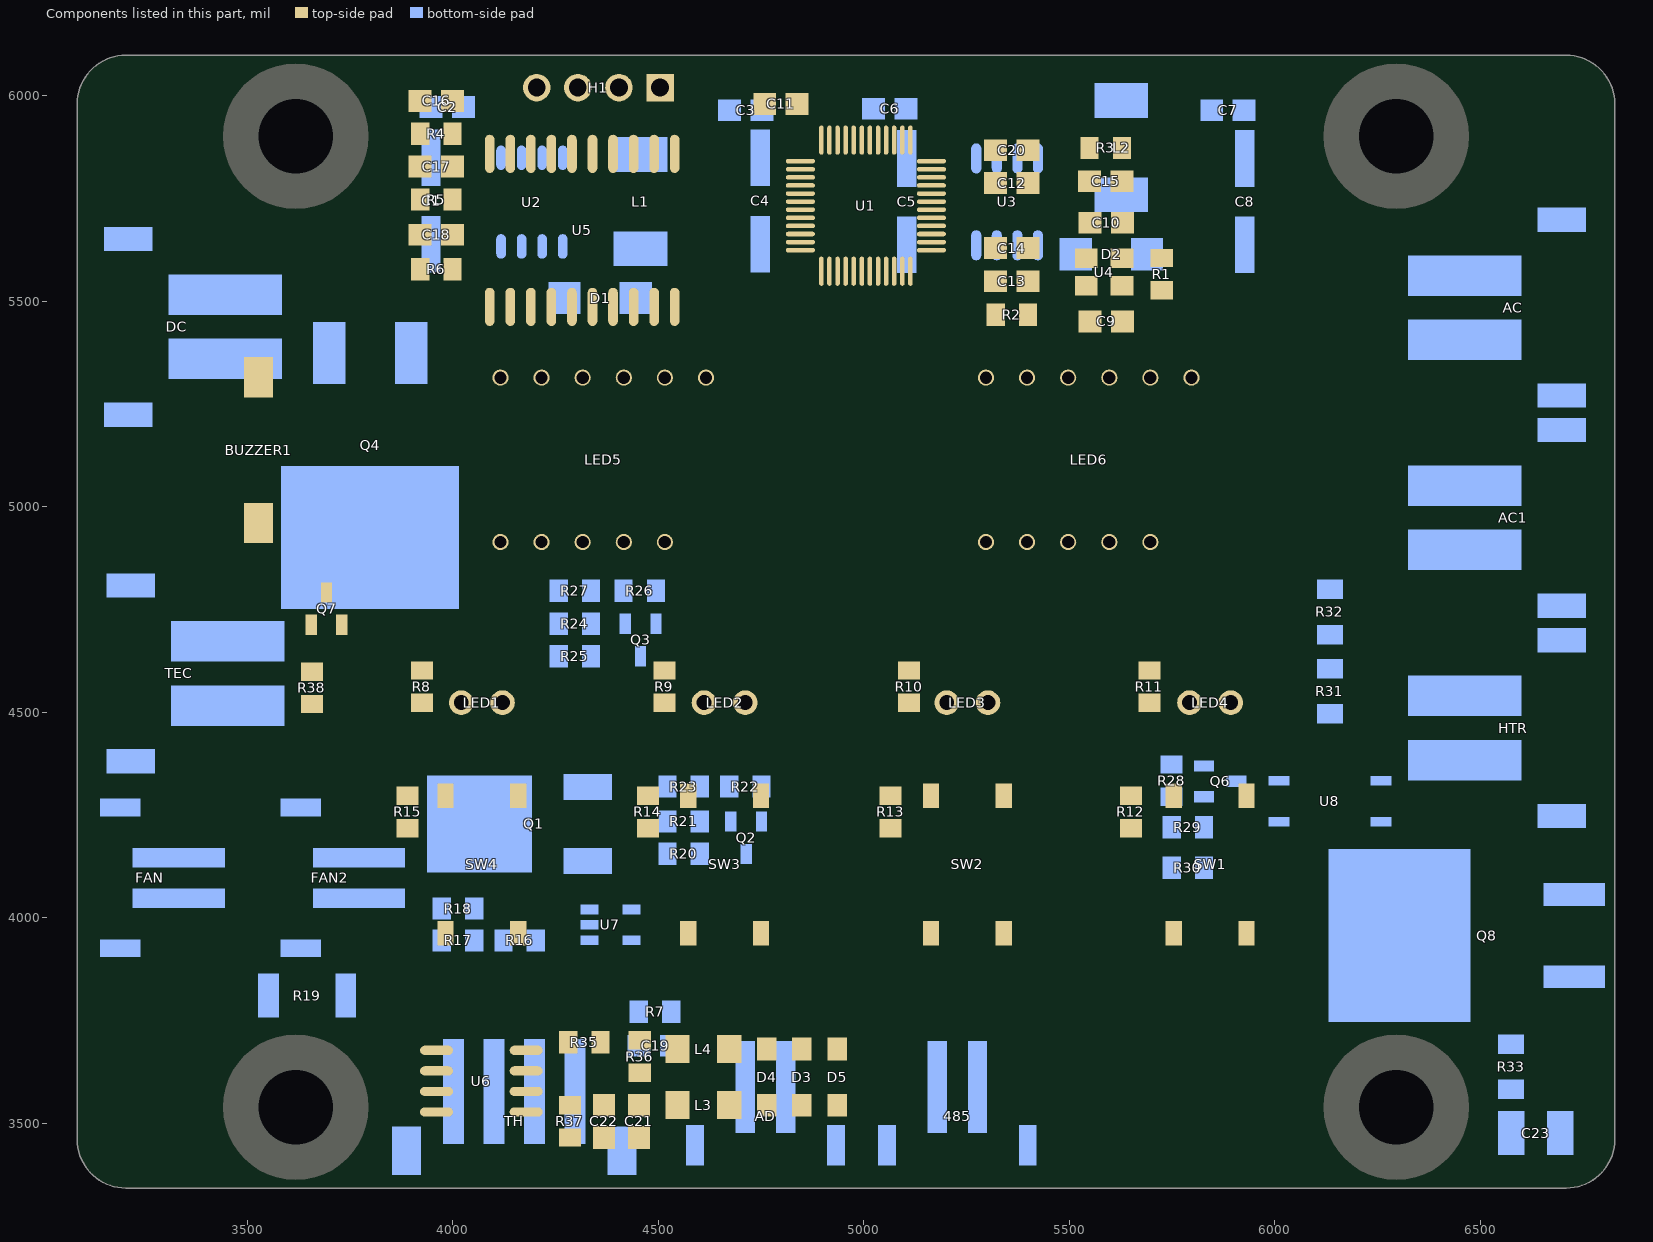
[diagram p0: the components of this part, seen from the top]
# Altium PCB MISC82750.pcbdoc (part 3 of 3)
Units mil, origin at the board's own origin, x right, y up, seen from the top; angles counter-clockwise.
Board outline 3740.2 x 2755.9 mil, 2 copper layers (Top Layer, Bottom Layer), stack 62.2 mil thick; 106 components, 84 nets, 362 pads, 334 vias.

## Silkscreen, mask and mechanical layers (free items; w line width, h text height) (continued)
Bottom Solder Mask Layer:
  lines w39.4: 3145.7,4875.6 3145.7,5151.2 ; 3145.7,5303.1 3145.7,5578.7 ; 3151.6,4460.1 3151.6,4735.7 ; 3153.5,3996.1 3153.5,4200.8 ; 3154.3,3493.7 3350.4,3493.7 ; 3154.3,3589.4 3350.4,3589.4 ; 3154.3,3705.2 3350.4,3705.2 ; 3154.3,3809.4 3470.6,3809.4 ; 3224.4,4875.6 3224.4,5151.2 ; 3224.4,5303.1 3224.4,5578.7 ; 3230.3,4460.1 3230.3,4735.7 ; 3311,3929.1 3496.1,3929.1 ; 3334.6,4889.8 3334.6,5157.5 ; 3413.4,4208.7 3874,4208.7 ; 3413.4,4318.9 3873.5,4318.9 ; 3427.6,4889.8 3427.6,5158.8 ; 3492.1,4039.4 3602.4,4039.4 ; 3503.9,4145.7 3598.4,4145.7 ; 3610.2,5527.6 3881.9,5527.6 3901.6,5507.9 ; 3645.7,4677.2 3996.1,4677.2 ; 3850.4,3881.9 3850.4,3984.3